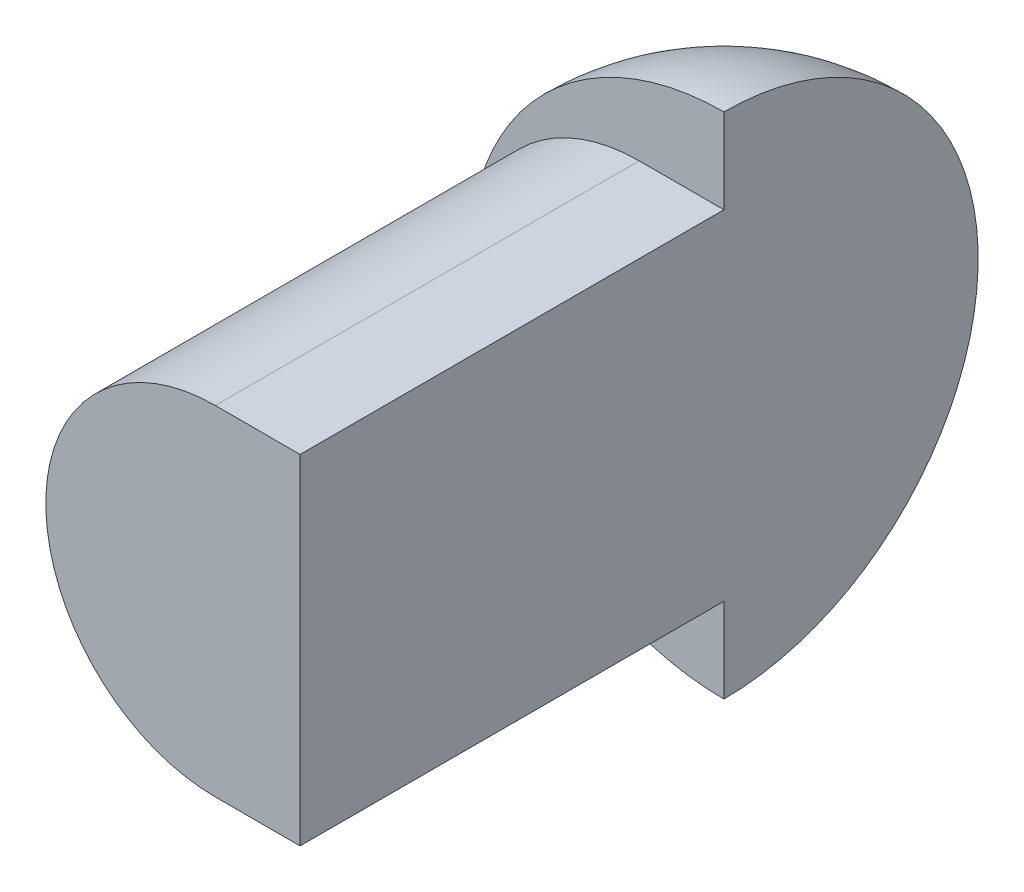
SolidWorks part; units mm, degrees
ref_plane "前视基准面" through (0, 0, 0) normal (0, 0, 1) x (1, 0, 0)
ref_plane "上视基准面" through (0, 0, 0) normal (0, 1, 0) x (1, 0, 0)
ref_plane "右视基准面" through (0, 0, 0) normal (1, 0, 0) x (0, 0, -1)
sketch "草图1" plane through (0, 0, 0) normal (0, 0, 1) x (1, 0, 0)
  line L0 (0, 0) -> (0, -80)
  line L1 (0, -80) -> (-20, -80)
  line L2 (-20, 0) -> (0, 0)
  arc A0 (-20, -80) -> (-20, 0) centre (-20, -40) cw
extrude "凸台-拉伸1" add sketch "草图1" against normal blind 100
sketch3d "3D草图1"
  point P0 (0, -44.0413, -47.6259)
ref_plane "基准面1" through (0, 0, 0) normal (1, 0, 0) x (0, 0, -1)
sketch "草图2" plane through (0, 0, 0) normal (1, 0, 0) x (0, 0, -1)
  line L0 (100, -80) -> (100, 0) construction
  line L1 (100, 20) -> (100, -100)
  arc A0 (100, 20) -> (100, -100) centre (100, -40) cw
revolve "旋转1" add sketch "草图2" angle 90 about L1
